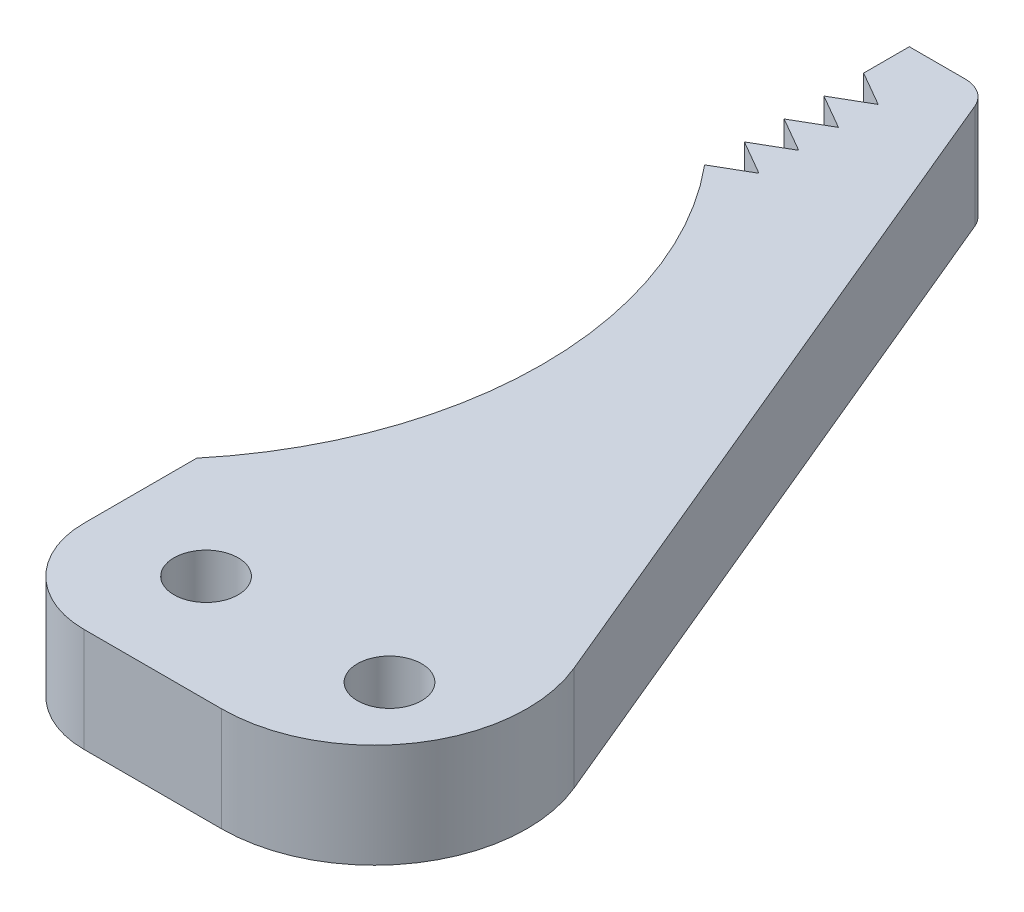
from build123d import *

# Parameters (mm, degrees)
BOSS_EXTRUDE1_DEPTH = 8.636
SKETCH3_R           = 2.667
CUT_EXTRUDE1_DEPTH  = 19.05
FILLET1_R           = 12.7
FILLET2_R           = 2.54
FILLET3_R           = 7.62
CUT_EXTRUDE2_DEPTH  = 84.000499974
SCALE1_SCALE        = 2


with BuildPart() as part:
    # Sketch1 → Boss-Extrude1 (new body)
    with BuildSketch(Plane(origin=(0, 0, 0), x_dir=(1, 0, 0), z_dir=(0, 1, 0))):
        with BuildLine():
            Line((0, 0), (38.1, 0))
            Line((38.1, 0), (6.35, 76.2))
            Line((6.35, 76.2), (0, 76.2))
            Line((0, 76.2), (0, 59.198824612))
            ThreePointArc((0, 59.198824612), (7.62, 38.1), (0, 17.001175388))
            Line((0, 17.001175388), (0, 0))
        make_face()
    extrude(amount=BOSS_EXTRUDE1_DEPTH)

    # Sketch3 → Cut-Extrude1 (cut)
    with BuildSketch(Plane(origin=(0, 8.636, 0), x_dir=(1, 0, 0), z_dir=(0, 1, 0))):
        with Locations(Location((8.89, 8.89, 0), (0, 0, 270))):
            Circle(SKETCH3_R)
        with Locations(Location((24.13, 8.89, 0), (0, 0, 270))):
            Circle(SKETCH3_R)
    extrude(amount=-CUT_EXTRUDE1_DEPTH, mode=Mode.SUBTRACT)

    # Fillet1
    fillet1_edges = [part.edges().sort_by_distance(p)[0] for p in [
        (38.1, 4.318, 0),
    ]]
    fillet(fillet1_edges, radius=FILLET1_R)

    # Fillet2
    fillet2_edges = [part.edges().sort_by_distance(p)[0] for p in [
        (6.35, 4.318, -76.2),
    ]]
    fillet(fillet2_edges, radius=FILLET2_R)

    # Fillet3
    fillet3_edges = [part.edges().sort_by_distance(p)[0] for p in [
        (0, 4.318, 0),
    ]]
    fillet(fillet3_edges, radius=FILLET3_R)

    # Sketch4 → Cut-Extrude2 (cut, through all)
    with BuildSketch(Plane(origin=(0, 8.636, 0), x_dir=(1, 0, 0), z_dir=(0, 1, 0))):
        Polygon((0, 62.500824612), (0, 59.198824612), (2.859615883, 60.849824612), align=None)
        Polygon((0, 65.802824612), (0, 62.500824612), (2.859615883, 64.151824612), align=None)
        Polygon((0, 69.104824612), (0, 65.802824612), (2.859615883, 67.453824612), align=None)
        Polygon((0, 72.406824612), (0, 69.104824612), (2.859615883, 70.755824612), align=None)
    extrude(amount=-CUT_EXTRUDE2_DEPTH, mode=Mode.SUBTRACT)


with BuildPart() as part_1:
    # Scale1: scaled about (0, 0, 0)
    add(part.part.scale(SCALE1_SCALE))


solid = part_1.part
